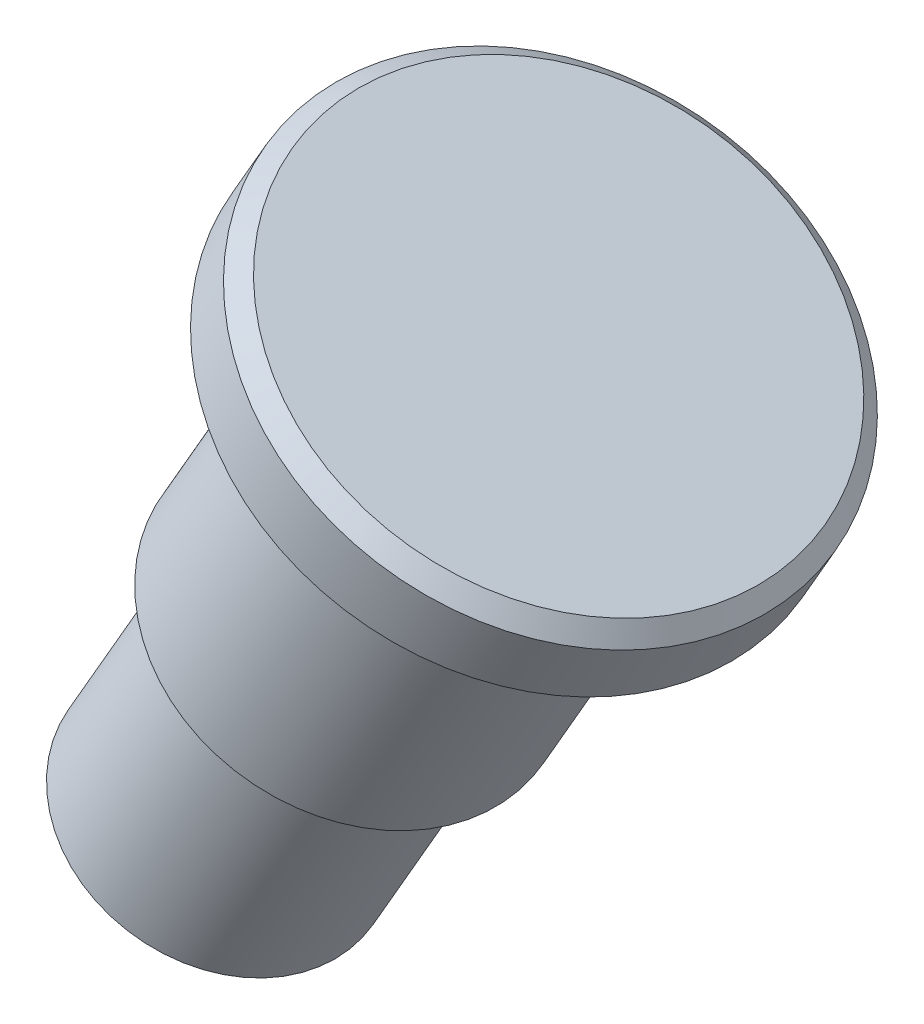
SolidWorks part; units mm, degrees
material "Q235B"
ref_plane "Front Plane" through (0, 0, 0) normal (0, 0, 1) x (1, 0, 0)
ref_plane "Top Plane" through (0, 0, 0) normal (0, 1, 0) x (1, 0, 0)
ref_plane "Right Plane" through (0, 0, 0) normal (1, 0, 0) x (0, 0, -1)
sketch "Sketch1" plane through (0, 0, 0) normal (0, 0, 1) x (1, 0, 0)
  line L0 (-91.125, 38.895) -> (-85.325, 48.9409) construction
  line L1 (-101.9503, 45.145) -> (-80.2997, 32.645) construction
  line L2 (-98.3154, 56.4409) -> (-72.3346, 41.4409) construction
  line L4 (-80.9949, 46.4409) -> (-78.8298, 45.1909)
  line L5 (-78.8298, 45.1909) -> (-77.3298, 47.7889)
  line L6 (-77.3298, 47.7889) -> (-83.825, 51.5389)
  line L7 (-85.325, 48.9409) -> (-83.825, 51.5389) construction
  line L8 (-80.9949, 46.4409) -> (-85.9949, 37.7806)
  line L9 (-86.7949, 36.395) -> (-83.9949, 41.2447) construction
  line L10 (-85.9949, 37.7806) -> (-86.8609, 38.2806)
  line L11 (-86.8609, 38.2806) -> (-90.8609, 31.3524)
  line L12 (-90.8609, 31.3524) -> (-94.325, 33.3524)
  line L13 (-91.125, 38.895) -> (-94.325, 33.3524) construction
  line L14 (-83.825, 51.5389) -> (-94.325, 33.3524)
  dimension "D1" = 3
  dimension "D2" = 15
  dimension "D3" = 10
  dimension "D4" = 8
  dimension "D5" = 8
revolve "Revolve1" add sketch "Sketch1" angle 360 about L14
cosmetic thread "Cosmetic Thread1" parameters "D2"=6.647
chamfer "Chamfer1" distance 0.5 angle 45 4 edges at (-90.3202, 55.2889, 0) (-91.8202, 52.6909, 0) (-94.6551, 42.7806, 0) (-97.7891, 35.3524, 0)
